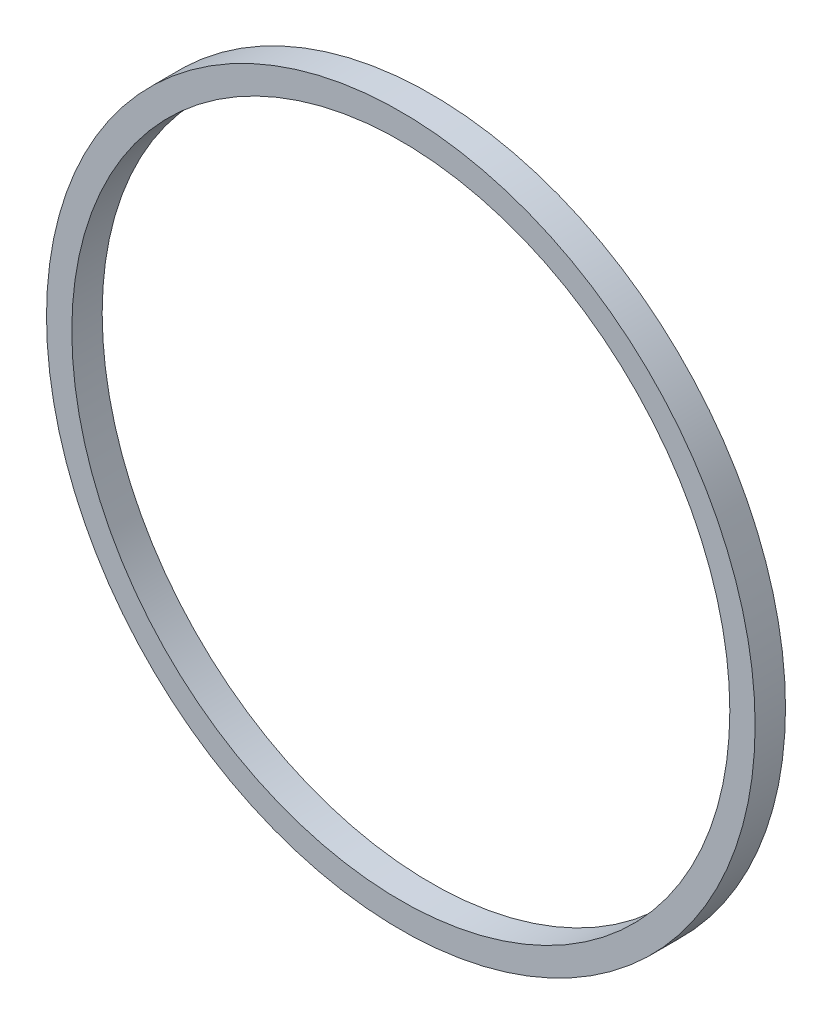
from build123d import *

# Parameters (mm, degrees)
SKETCH_1_R      = 35
SKETCH_1_R_2    = 32.5
EXTRUDE_1_DEPTH = 3


with BuildPart() as part:
    # 草图1 → 凸台-拉伸1 (new body)
    with BuildSketch(Plane.XY):
        Circle(SKETCH_1_R)
        Circle(SKETCH_1_R_2, mode=Mode.SUBTRACT)
    extrude(amount=EXTRUDE_1_DEPTH)


solid = part.part
